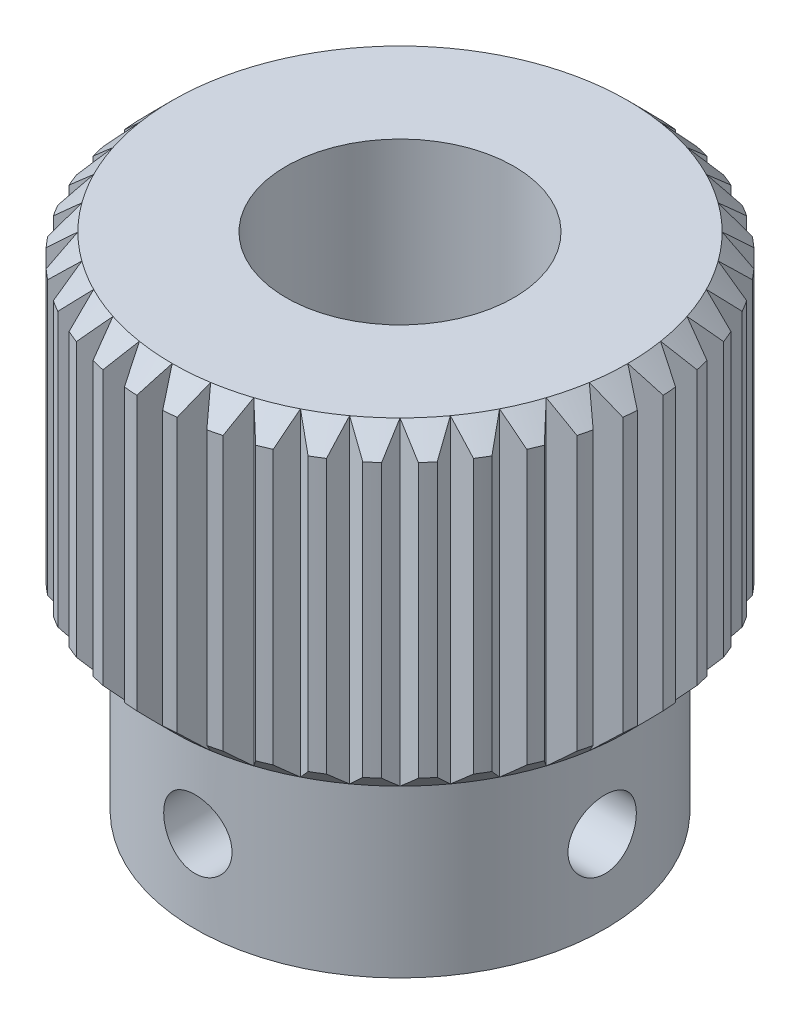
from build123d import *

# Parameters (mm, degrees)
CUT_EXTRUDE1_DEPTH = 14.472193585
CIRPATTERN1_COUNT  = 40
SKETCH3_R          = 0.75
CUT_EXTRUDE2_DEPTH = 10
SKETCH4_R          = 0.75
CUT_EXTRUDE3_DEPTH = 10


with BuildPart() as part:
    # Sketch1 → Revolve1 (revolve)
    with BuildSketch(Plane.XY, mode=Mode.PRIVATE) as revolve1_sk:
        Polygon((2.5, 0), (2.5, 11), (5, 11), (5.5, 10.5), (5.5, 4.5), (5, 4), (4.5, 4), (4.5, 0), align=None)
    revolve(revolve1_sk.sketch.rotate(Axis((0, 0, 0), (0, 1, 0)), 90), axis=Axis((0, 0, 0), (0, 1, 0)))

    # Sketch2 → Cut-Extrude1 (cut, through all)
    with BuildSketch(Plane(origin=(0, 11, 0), x_dir=(1, 0, 0), z_dir=(0, 1, 0))):
        Polygon((0.433012702, 5.75), (-0.433012702, 5.75), (0, 5), align=None)
    cut_extrude1 = extrude(amount=-CUT_EXTRUDE1_DEPTH, mode=Mode.SUBTRACT)

    # CirPattern1: Cut-Extrude1 ×40 about axis
    cirpattern1_axis = Axis((0, 0, 0), (0, 1, 0))
    for i in range(1, CIRPATTERN1_COUNT):
        add(cut_extrude1.rotate(cirpattern1_axis, i * 360 / CIRPATTERN1_COUNT), mode=Mode.SUBTRACT)

    # Sketch3 → Cut-Extrude2 (cut)
    with BuildSketch(Plane.XY):
        with Locations(Location((0, 1.804360247, 0), (0, 0, 180))):
            Circle(SKETCH3_R)
    extrude(amount=CUT_EXTRUDE2_DEPTH, mode=Mode.SUBTRACT)

    # Sketch4 → Cut-Extrude3 (cut)
    with BuildSketch(Plane(origin=(0, 0, 0), x_dir=(0, 0, -1), z_dir=(1, 0, 0))):
        with Locations(Location((0, 1.8, 0), (0, 0, 180))):
            Circle(SKETCH4_R)
    extrude(amount=CUT_EXTRUDE3_DEPTH, mode=Mode.SUBTRACT)


solid = part.part
